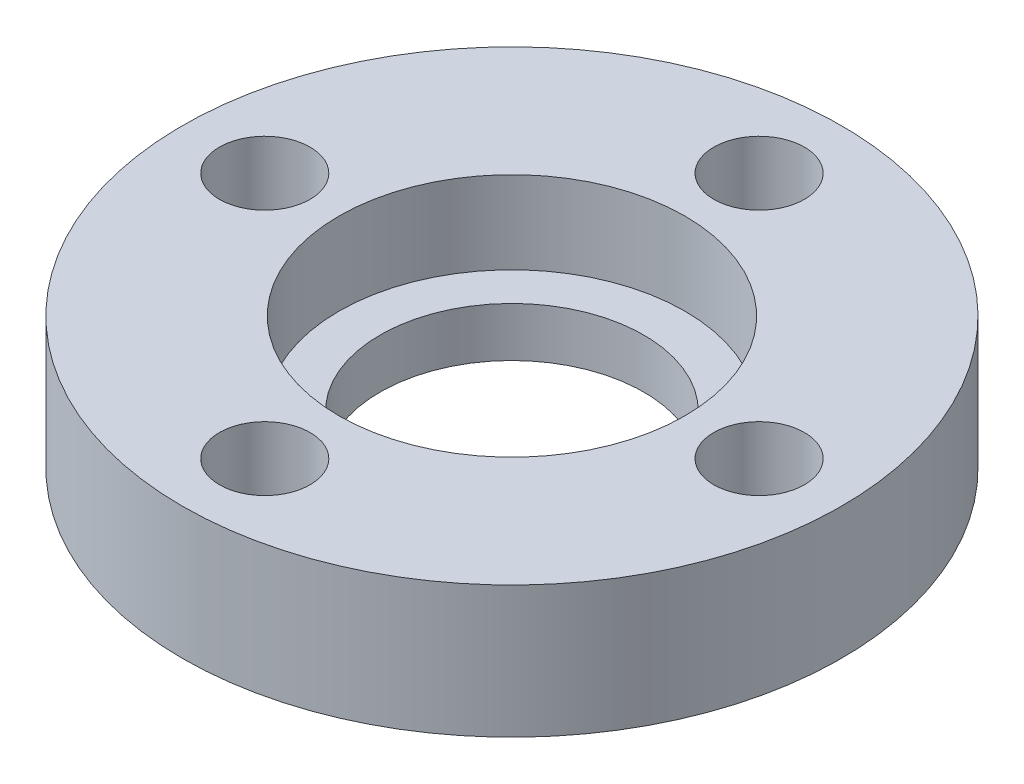
from build123d import *

# Parameters (mm, degrees)
SKETCH1_R                 = 40
SKETCH1_R_2               = 16
BOSS_EXTRUDE1_DEPTH       = 16
SKETCH2_R                 = 21
CUT_EXTRUDE1_DEPTH        = 10
M10_CLEARANCE_HOLE1_D     = 11
M10_CLEARANCE_HOLE1_DEPTH = 29.25
M10_CLEARANCE_HOLE1_TIP   = 3.304733405


with BuildPart() as part:
    # Sketch1 → Boss-Extrude1 (new body)
    with BuildSketch(Plane(origin=(0, 0, 0), x_dir=(1, 0, 0), z_dir=(0, 1, 0))):
        with Locations(Location((0, 0, 0), (0, 0, 270))):
            Circle(SKETCH1_R)
        with Locations(Location((0, 0, 0), (0, 0, 270))):
            Circle(SKETCH1_R_2, mode=Mode.SUBTRACT)
    extrude(amount=BOSS_EXTRUDE1_DEPTH)

    # Sketch2 → Cut-Extrude1 (cut)
    with BuildSketch(Plane(origin=(0, 16, 0), x_dir=(1, 0, 0), z_dir=(0, 1, 0))):
        with Locations(Location((0, 0, 0), (0, 0, 270))):
            Circle(SKETCH2_R)
    extrude(amount=-CUT_EXTRUDE1_DEPTH, mode=Mode.SUBTRACT)

    # M10 Clearance Hole1
    with Locations(Plane(origin=(0, 16, 0), x_dir=(1, 0, 0), z_dir=(0, 1, 0))):
        with Locations((0, -30), (0, 30), (-30, 0), (30, 0)):
            Hole(M10_CLEARANCE_HOLE1_D / 2, depth=M10_CLEARANCE_HOLE1_DEPTH)
            with Locations((0, 0, -(M10_CLEARANCE_HOLE1_DEPTH + M10_CLEARANCE_HOLE1_TIP / 2))):  # 118° drill point
                Cone(0, M10_CLEARANCE_HOLE1_D / 2, M10_CLEARANCE_HOLE1_TIP, mode=Mode.SUBTRACT)


solid = part.part
